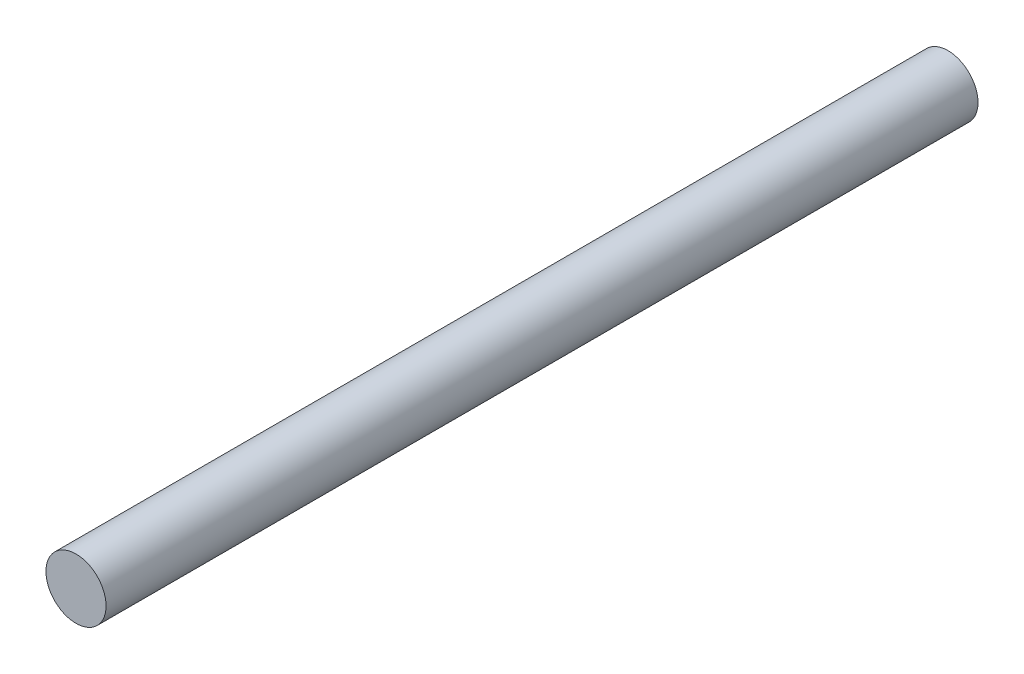
from build123d import *

# Parameters (mm, degrees)
SKETCH_1_R      = 10
EXTRUDE_1_DEPTH = 145


with BuildPart() as part:
    # 草图1 → 凸台-拉伸1 (new, symmetric)
    with BuildSketch(Plane.XY):
        Circle(SKETCH_1_R)
    extrude(amount=EXTRUDE_1_DEPTH, both=True)


solid = part.part
